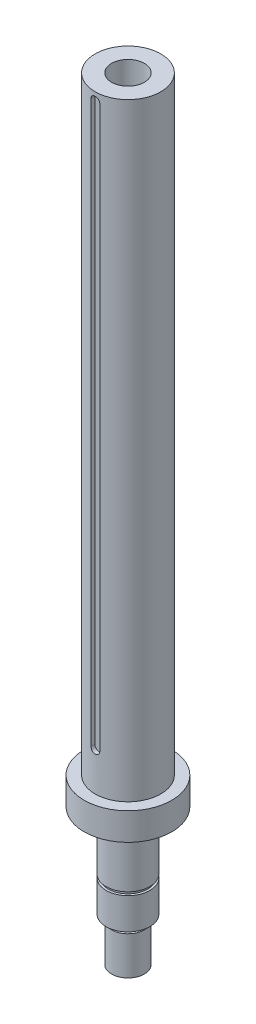
SolidWorks part; units mm, degrees
ref_plane "前视基准面" through (0, 0, 0) normal (0, 0, 1) x (1, 0, 0)
ref_plane "上视基准面" through (0, 0, 0) normal (0, 1, 0) x (1, 0, 0)
ref_plane "右视基准面" through (0, 0, 0) normal (1, 0, 0) x (0, 0, -1)
sketch "草图1" plane through (0, 0, 0) normal (0, 0, 1) x (1, 0, 0)
  line L0 (0, 247.8602) -> (0, -291.3817) construction
  line L1 (0, -243.6142) -> (15, -243.6142)
  line L2 (15, -243.6142) -> (15, -208.6142)
  line L3 (15, -208.6142) -> (10, -208.6142)
  line L4 (10, -208.6142) -> (10, -203.6142)
  line L5 (10, -203.6142) -> (20, -203.6142)
  line L6 (20, -203.6142) -> (20, -174.9142)
  line L7 (20, -174.9142) -> (18, -174.9142)
  line L8 (18, -174.9142) -> (18, -171.9142)
  line L9 (18, -171.9142) -> (20, -171.9142)
  line L10 (20, -171.9142) -> (20, -118.6142)
  line L11 (20, -118.6142) -> (40, -118.6142)
  line L12 (40, -118.6142) -> (40, -93.6142)
  line L13 (40, -93.6142) -> (30, -93.6142)
  line L14 (30, -93.6142) -> (30, 461.9758)
  line L15 (30, 461.9758) -> (0, 461.9758)
  line L16 (0, 461.9758) -> (0, -243.6142)
  dimension "D1" = 705.59
  dimension "D2" = 30
  dimension "D3" = 15
  dimension "D4" = 40
  dimension "D5" = 20
  dimension "D6" = 18
  dimension "D7" = 20
  dimension "D8" = 10
  dimension "D9" = 35
  dimension "D10" = 5
  dimension "D11" = 25
  dimension "D12" = 53.3
  dimension "D13" = 3
  dimension "D14" = 28.7
revolve "旋转1" add sketch "草图1" angle 360 about L0
sketch "草图2" plane through (0, 461.9758, 0) normal (0, 1, 0) x (1, 0, 0)
  circle A0 centre (0, 0) radius 15
  dimension "D1" = 30
extrude "切除-拉伸1" cut sketch "草图2" against normal blind 50
sketch "草图3" plane through (0, 461.9758, 0) normal (0, 1, 0) x (1, 0, 0)
  line L0 (0, 50.0925) -> (0, -47.0999) construction
  line L1 (-4, -29.7321) -> (4, -29.7321) construction
  line L3 (-4, -26.2321) -> (4, -26.2321)
  line L4 (-4, -26.2321) -> (-4, -33.2321)
  line L5 (-4, -33.2321) -> (4, -33.2321)
  line L6 (4, -26.2321) -> (4, -33.2321)
  line L7 (-4, -26.2321) -> (4, -33.2321) construction
  line L8 (-4, -33.2321) -> (4, -26.2321) construction
  circle A0 centre (0, 0) radius 30 construction
  circle A1 centre (0, 0) radius 30 construction
  point P8 (0, -29.7321)
  dimension "D1" = 8
  dimension "D2" = 7
  dimension "D3" = 8
  dimension "D4" = 3.5
extrude "切除-拉伸2" cut sketch "草图3" against normal blind 512.59 from offset 7.5 offset against normal yes
sketch "草图4" plane through (0, 0, 26.2321) normal (0, 0, 1) x (1, 0, 0)
  line L0 (4, -58.1142) -> (-4, -58.1142) construction
  line L2 (4, 454.4758) -> (-4, 454.4758) construction
  line L3 (-4, 454.4758) -> (4, 454.4758) construction
  line L4 (4, -58.1142) -> (-4, -58.1142) construction
  line L5 (4, -58.1142) -> (-4, -58.1142)
  line L6 (-4, 454.4758) -> (4, 454.4758)
  arc A0 (4, -58.1142) -> (-4, -58.1142) centre (0, -58.1142) cw
  arc A1 (-4, 454.4758) -> (4, 454.4758) centre (0, 454.4758) cw
extrude "切除-拉伸3" cut sketch "草图4" along normal blind 7
